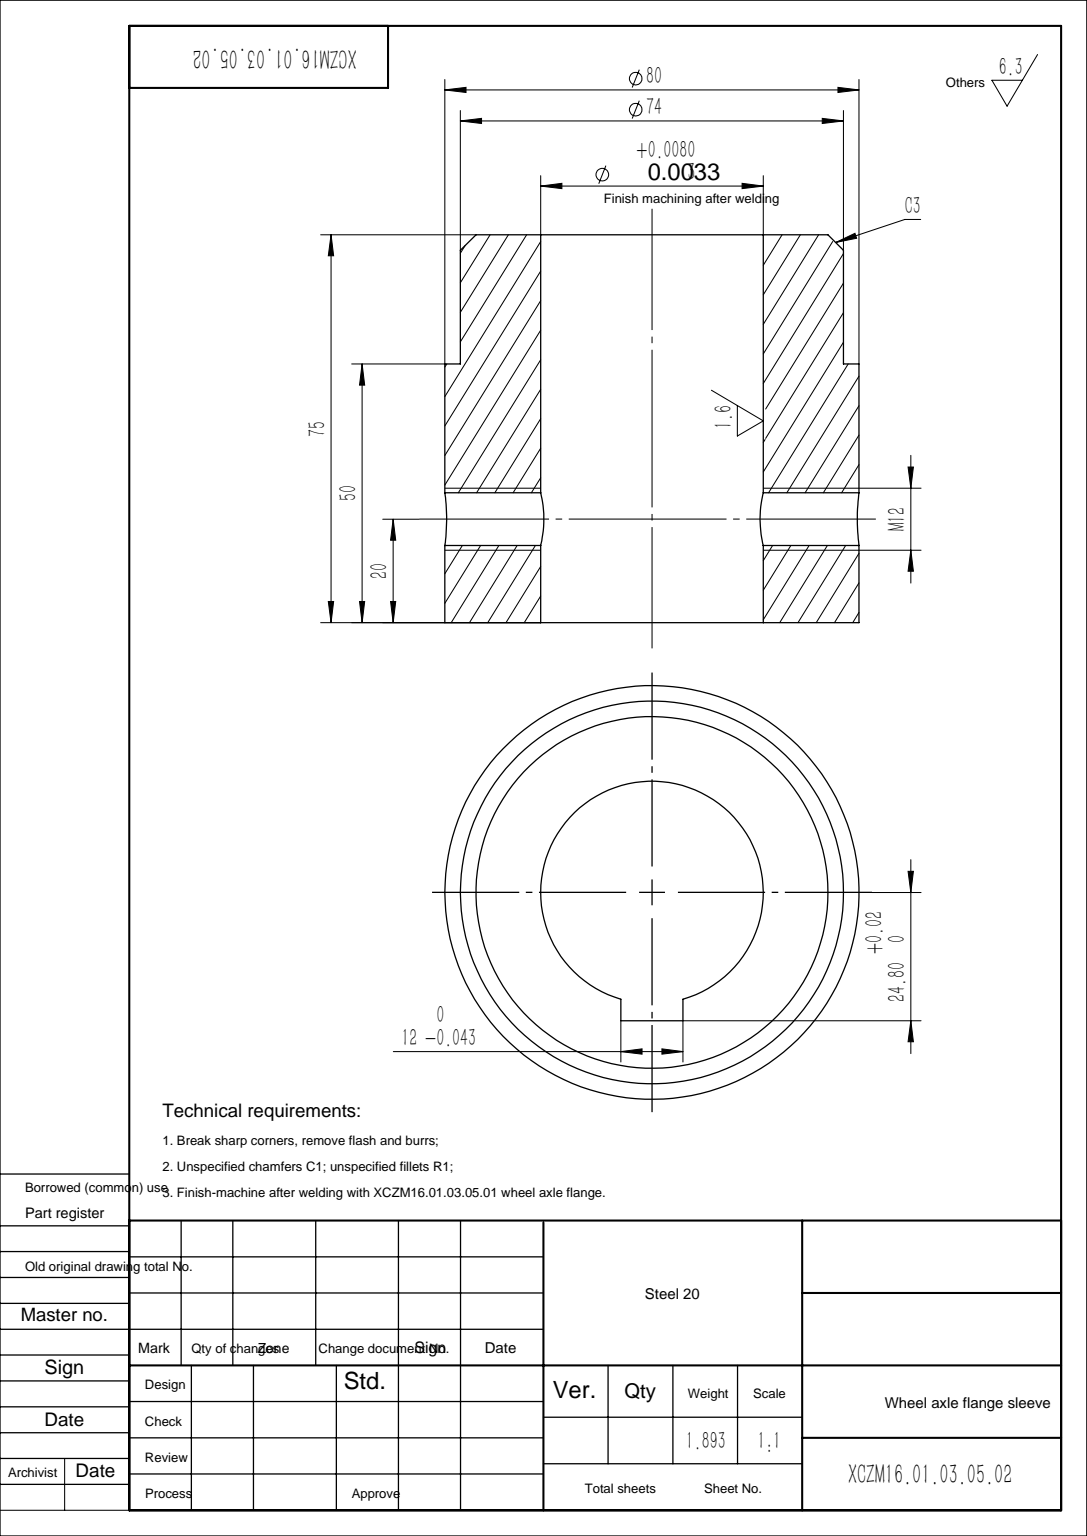
from build123d import *

# Parameters (mm, degrees)
CHAMFER1_SIZE      = 3
M12_TAPPED_HOLE1_D = 10.2
CUT_EXTRUDE1_REACH = 95.941
SKETCH6_W          = 12
SKETCH6_H          = 6.6


with BuildPart() as part:
    # Sketch2 → Revolve1 (revolve)
    with BuildSketch(Plane.XY, mode=Mode.PRIVATE) as revolve1_sk:
        Polygon((21.5, 75), (21.5, 0), (40, 0), (40, 50), (37, 50), (37, 75), align=None)
    revolve(revolve1_sk.sketch.rotate(Axis((0, 75, 0), (0, -1, 0)), 180), axis=Axis((0, 75, 0), (0, -1, 0)))

    # Chamfer1
    chamfer1_edges = [part.edges().sort_by_distance(p)[0] for p in [
        (37, 75, 0),
    ]]
    chamfer(chamfer1_edges, length=CHAMFER1_SIZE)

    # M12 Tapped Hole1 (through all)
    with Locations(Plane(origin=(40, 0, 0), x_dir=(0, 0, -1), z_dir=(1, 0, 0))):
        with Locations((0, 20)):
            Hole(M12_TAPPED_HOLE1_D / 2)

    # Sketch6 → Cut-Extrude1 (cut, up to next)
    with BuildSketch(Plane(origin=(0, 75, 0), x_dir=(1, 0, 0), z_dir=(0, 1, 0)), mode=Mode.PRIVATE) as cut_extrude1_sk1:
        with Locations((0, -21.5)):
            Rectangle(SKETCH6_W, SKETCH6_H)
    cut_extrude1_tool1 = extrude(cut_extrude1_sk1.sketch, amount=-CUT_EXTRUDE1_REACH, mode=Mode.PRIVATE) & part.part
    add(cut_extrude1_tool1.solids().sort_by_distance((0, 75, 21.5))[0], mode=Mode.SUBTRACT)


solid = part.part
